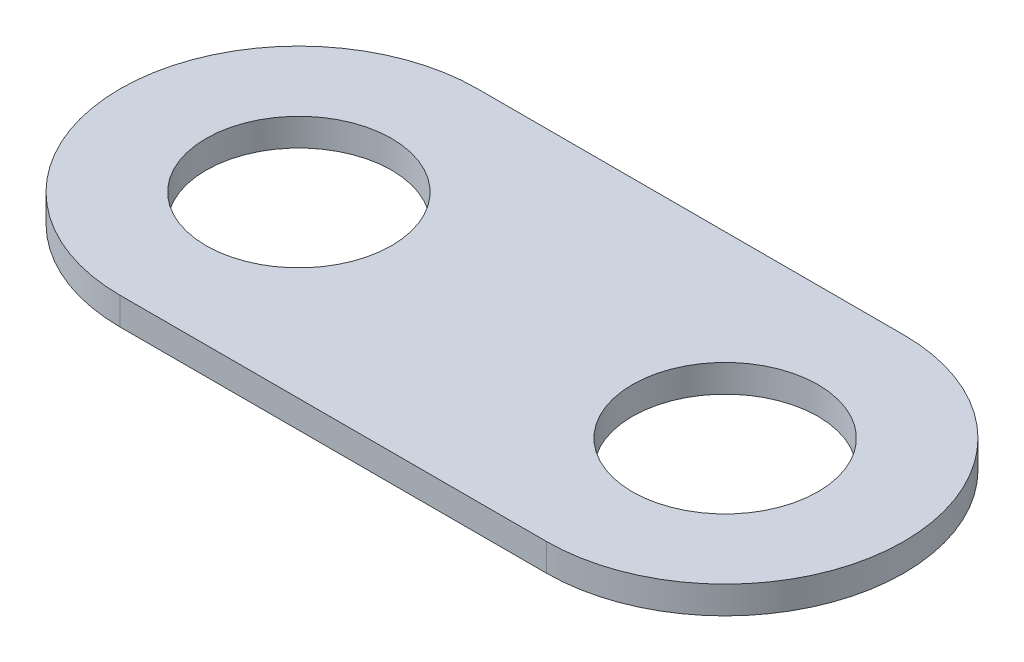
SolidWorks part; units mm, degrees
material "Q235A"
ref_plane "Front" through (0, 0, 0) normal (0, 0, 1) x (1, 0, 0)
ref_plane "Top" through (0, 0, 0) normal (0, 1, 0) x (1, 0, 0)
ref_plane "Right" through (0, 0, 0) normal (1, 0, 0) x (0, 0, -1)
sketch "Sketch1" plane through (0, 0, 0) normal (0, 1, 0) x (1, 0, 0)
  line L0 (-62, 26) -> (0, 26)
  line L3 (0, -26) -> (-62, -26)
  circle A0 centre (0, 0) radius 13.5
  circle A1 centre (-62, 0) radius 13.5
  arc A2 (-62, 26) -> (-62, -26) centre (-62, 0) ccw
  arc A3 (0, -26) -> (0, 26) centre (0, 0) ccw
  circle A4 centre (0, 0) radius 26 construction
  circle A5 centre (-62, 0) radius 26 construction
  dimension "D1" = 27
  dimension "D2" = 62
  dimension "D3" = 52
extrude "Extrude1" add sketch "Sketch1" along normal mid plane 4
